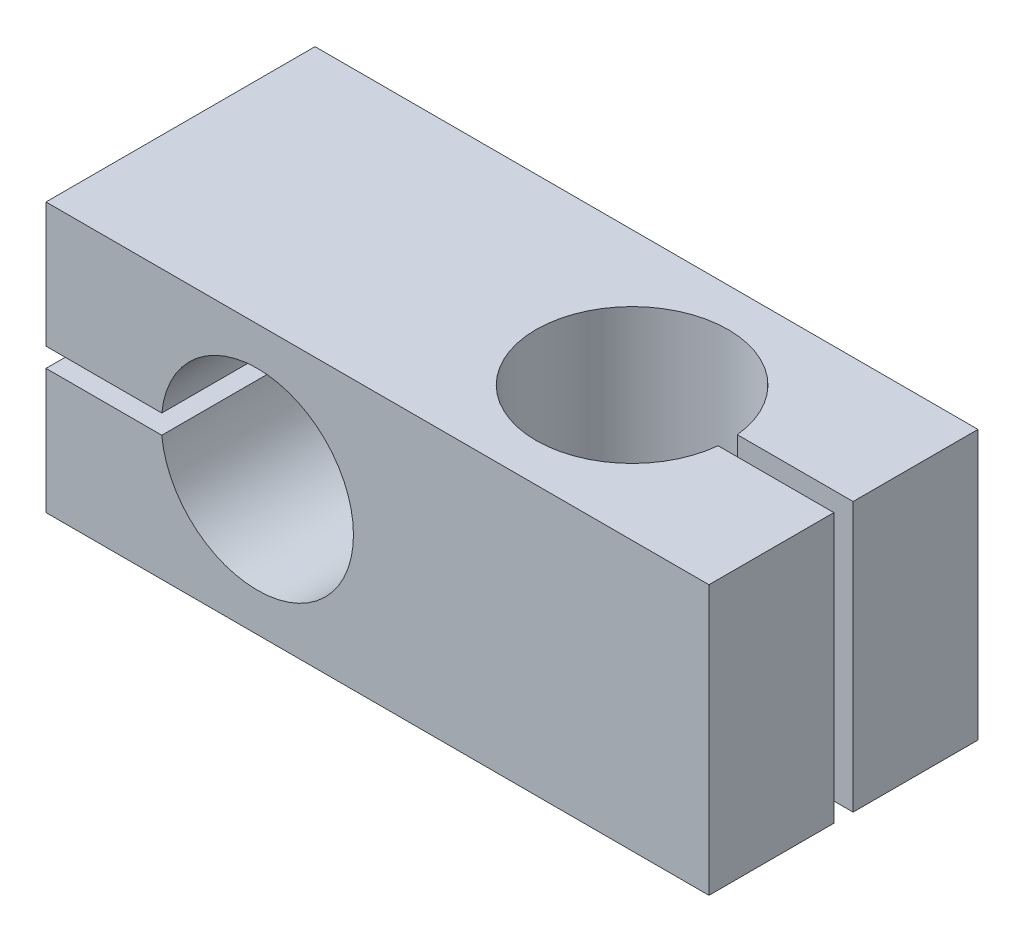
from build123d import *

# Parameters (mm, degrees)
SKETCH_1_W          = 69
SKETCH_1_H          = 28
EXTRUDE_1_DEPTH     = 14
CUT_EXTRUDE_1_DEPTH = 47.585942086
CUT_EXTRUDE_2_DEPTH = 47.585942086


with BuildPart() as part:
    # 草图1 → 凸台-拉伸1 (new, symmetric)
    with BuildSketch(Plane.XY):
        Rectangle(SKETCH_1_W, SKETCH_1_H)
    extrude(amount=EXTRUDE_1_DEPTH, both=True)

    # 草图2 → 切除-拉伸1 (cut, through all)
    with BuildSketch(Plane.XY.offset(14)):
        with BuildLine():
            Line((-34.5, 1), (-22.449874371, 1))
            ThreePointArc((-22.449874371, 1), (-2.5, 0), (-22.449874371, -1))
            Line((-22.449874371, -1), (-34.5, -1))
            Line((-34.5, -1), (-34.5, 1))
        make_face()
    extrude(amount=-CUT_EXTRUDE_1_DEPTH, mode=Mode.SUBTRACT)

    # 草图3 → 切除-拉伸2 (cut, through all)
    with BuildSketch(Plane(origin=(0, 14, 0), x_dir=(1, 0, 0), z_dir=(0, 1, 0))):
        with BuildLine():
            Line((22.449874371, -1), (34.5, -1))
            Line((34.5, -1), (34.5, 1))
            Line((34.5, 1), (22.449874371, 1))
            ThreePointArc((22.449874371, 1), (2.5, 0), (22.449874371, -1))
        make_face()
    extrude(amount=-CUT_EXTRUDE_2_DEPTH, mode=Mode.SUBTRACT)


solid = part.part
